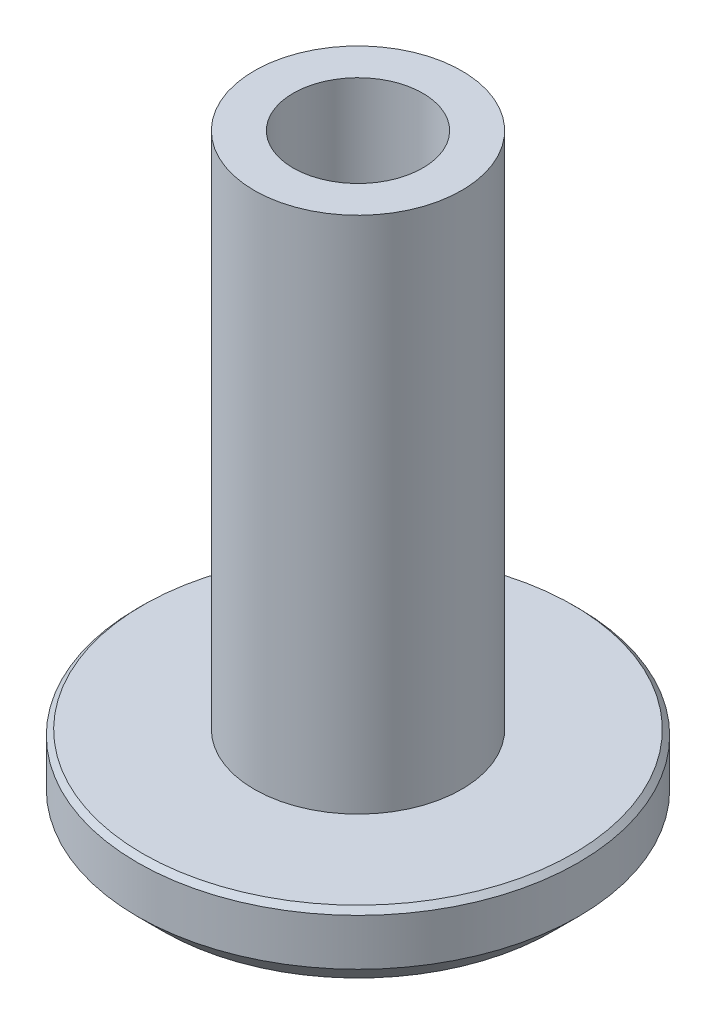
SolidWorks part; units mm, degrees
material "AISI 304"
ref_plane "前视基准面" through (0, 0, 0) normal (0, 0, 1) x (1, 0, 0)
ref_plane "上视基准面" through (0, 0, 0) normal (0, 1, 0) x (1, 0, 0)
ref_plane "右视基准面" through (0, 0, 0) normal (1, 0, 0) x (0, 0, -1)
sketch "草图1" plane through (0, 0, 0) normal (0, 1, 0) x (1, 0, 0)
  circle A0 centre (0, 0) radius 4.25
  dimension "D1" = 8.5
extrude "凸台-拉伸1" add sketch "草图1" along normal blind 1.5
sketch "草图2" plane through (0, 1.5, 0) normal (0, 1, 0) x (1, 0, 0)
  circle A0 centre (0, 0) radius 2
  dimension "D1" = 4
extrude "凸台-拉伸2" add sketch "草图2" along normal blind 10
hole_wizard "M3 螺纹孔1" positions "草图6" profile "草图5" tap size "M3" standard "GB"
sketch "草图6" plane through (0, 11.5, 0) normal (0, 1, 0) x (1, 0, 0)
  point P0 (0, 0)
sketch "草图5" plane through (0, 11.5, 0) normal (1, 0, 0) x (0, 0, 1)
  line L0 (0, 0) -> (0, 9.2511)
  line L1 (0, 9.2511) -> (1.25, 8.5)
  line L2 (1.25, 8.5) -> (1.25, 0)
  line L5 (1.25, 0) -> (0, 0)
  line L10 (0, 9.2511) -> (-1.25, 8.5) construction
  line L11 (0, -6.35) -> (0, 107.95) construction
  dimension "螺纹孔钻头直径" = 2.5
  dimension "螺纹孔钻头深度" = 8.5
  dimension "导头角度" = 118
cosmetic thread "孔螺纹线1" parameters "D1"=6, "D2"=3
sketch "草图7" plane through (0, 0, 0) normal (0, -1, 0) x (1, 0, 0)
  line L0 (0, 1.4434) -> (-1.25, 0.7217)
  line L1 (-1.25, 0.7217) -> (-1.25, -0.7217)
  line L2 (-1.25, -0.7217) -> (0, -1.4434)
  line L3 (0, -1.4434) -> (1.25, -0.7217)
  line L4 (1.25, -0.7217) -> (1.25, 0.7217)
  line L5 (1.25, 0.7217) -> (0, 1.4434)
  circle A0 centre (0, 0) radius 1.4434 construction
  dimension "D1" = 2.5
extrude "切除-拉伸1" cut sketch "草图7" against normal blind 1
chamfer "倒角1" distance 0.5 angle 45 1 edges at (0, 0, 4.25)
chamfer "倒角2" distance 0.1 angle 45 1 edges at (0, 1.5, 4.25)
